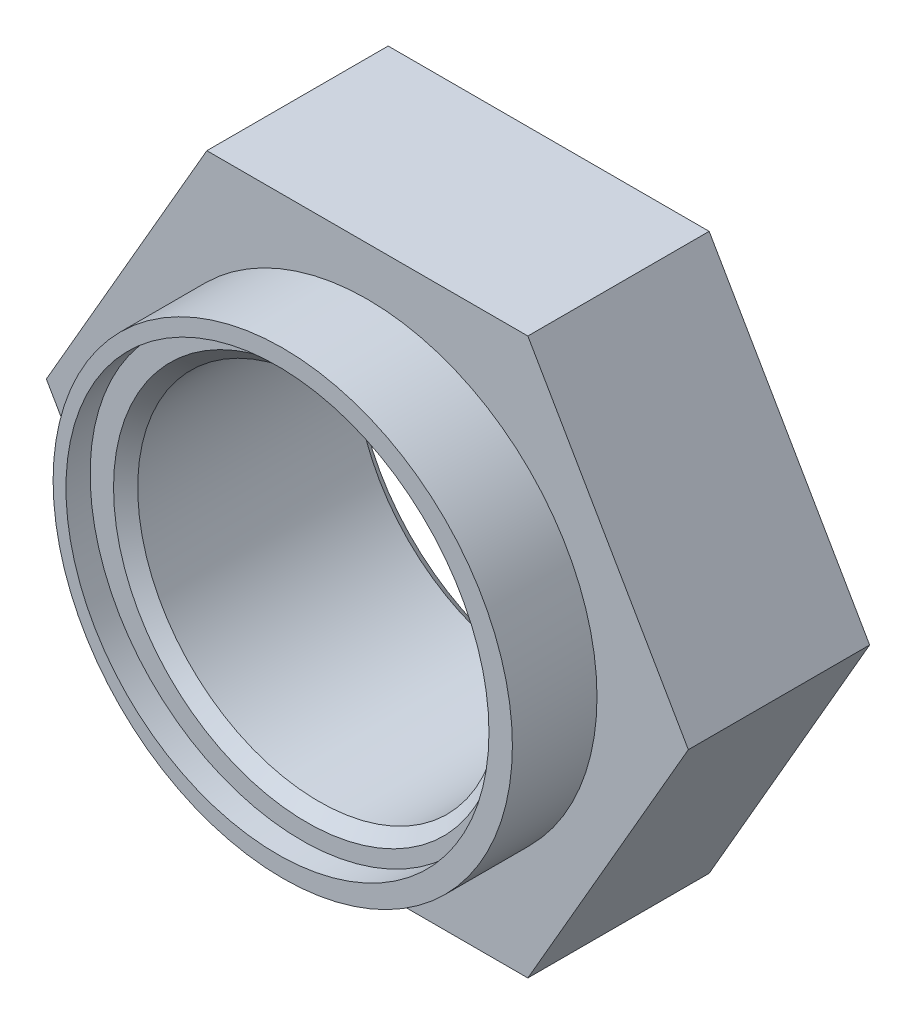
SolidWorks part; units mm, degrees
ref_plane "前视基准面" through (0, 0, 0) normal (0, 0, 1) x (1, 0, 0)
ref_plane "上视基准面" through (0, 0, 0) normal (0, 1, 0) x (1, 0, 0)
ref_plane "右视基准面" through (0, 0, 0) normal (1, 0, 0) x (0, 0, -1)
sketch "草图1" plane through (0, 0, 0) normal (0, 0, 1) x (1, 0, 0)
  circle A0 centre (0, 0) radius 19
  dimension "D1" = 38
extrude "凸台-拉伸1" add sketch "草图1" against normal blind 7
sketch "草图2" plane through (0, 0, -7) normal (0, 0, -1) x (-1, 0, 0)
  line L0 (-26.5581, 0) -> (26.5581, 0) construction
  line L1 (13.2791, -23) -> (26.5581, 0)
  line L2 (26.5581, 0) -> (13.2791, 23)
  line L3 (13.2791, 23) -> (-13.2791, 23)
  line L4 (-13.2791, 23) -> (-26.5581, 0)
  line L5 (-26.5581, 0) -> (-13.2791, -23)
  line L6 (-13.2791, -23) -> (13.2791, -23)
  circle A0 centre (0, 0) radius 23 construction
  dimension "D1" = 46
extrude "凸台-拉伸2" add sketch "草图2" along normal blind 15
sketch "草图3" plane through (0, 0, 0) normal (0, 0, 1) x (1, 0, 0)
  circle A0 centre (-0.4374, 0) radius 17.5
  dimension "D1" = 35
extrude "切除-拉伸1" cut sketch "草图3" against normal blind 2
sketch "草图4" plane through (0, 0, -2) normal (0, 0, 1) x (1, 0, 0)
  circle A0 centre (0, 0) radius 15
  dimension "D1" = 30
extrude "切除-拉伸2" cut sketch "草图4" against normal through all
cosmetic thread "装饰螺纹线1" parameters "D2"=90
chamfer "倒角1" distance 1 angle 45 2 edges at (15, 0, -22) (15, 0, -2)
